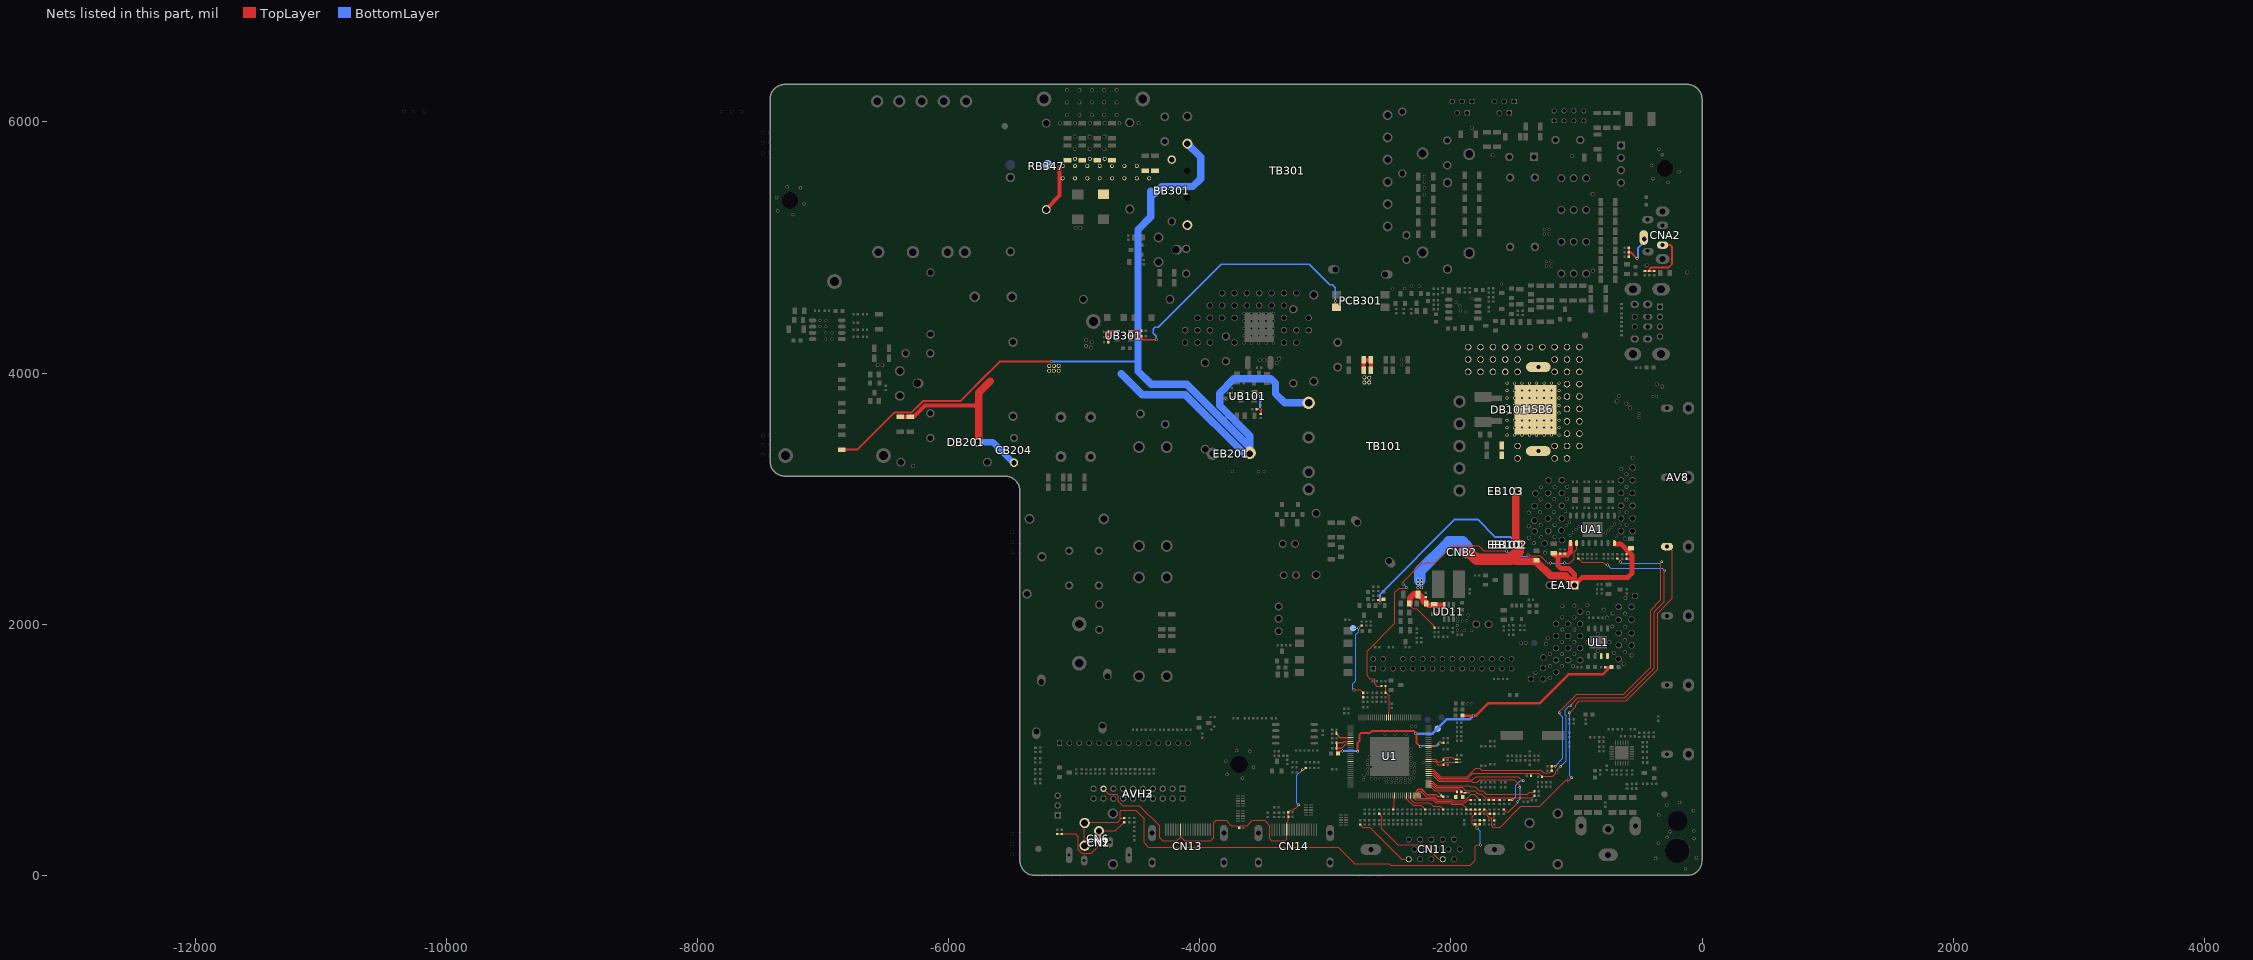
[diagram p0: the nets of this part, all layers, seen from the top]
# Altium PCB MISC84277.PcbDoc (part 7 of 15)
Units mil, origin at the board's own origin, x right, y up, seen from the top; angles counter-clockwise.
Board outline 7422.08 x 6299.21 mil, 2 copper layers (TopLayer, BottomLayer), stack 61.855 mil thick; 709 components, 395 nets, 2812 pads, 811 vias.

## Via types
v1: diameter 23.62, hole 15.75, TopLayer to BottomLayer, tented both sides, 437 vias
v2: diameter 19.68, hole 11.81, TopLayer to BottomLayer, tented both sides, 353 vias
v3: diameter 31.5, hole 23.62, TopLayer to BottomLayer, tented both sides, 16 vias
v4: diameter 31.5, hole 19.68, TopLayer to BottomLayer, tented both sides, 4 vias
v5: diameter 17.72, hole 9.84, TopLayer to BottomLayer, tented both sides, 1 vias

## Nets (pads, with @x,y where several pads share a name; then routed paths per layer and width w, separated by ;. In a path a pad name is that pad's centre, name@x,y a point inside that pad or via, vN(x,y) a via of type N, cw(c..) or ccw(c..) an arc to the next point about the centre after c; other vN are vias at no path point) (continued)
12V: C1.2 CA9.1 CA11.1 CA23.1 CA24.1 CD1.1 CD5.1 CD6.1 CD8.1 CD9.2 CD10.2 CNB2.2 DB101.2 EA1.1 EB101.1@-1464.92,2633.4 EB102.1@-1464.92,2633.4 EB103.1@-1465.89,3058.4 HSB6.1@-1304,3378.35 HSB6.2 pad.VIA5@-977.11,3419.43 pad.VIA5@-977.11,3517.85 pad.VIA5@-977.11,3616.28 pad.VIA5@-977.11,3714.7 pad.VIA5@-977.11,3813.13 pad.VIA5@-977.11,3911.55 pad.VIA5@-977.11,4009.98 pad.VIA5@-977.11,4108.4 pad.VIA5@-977.11,4206.83 pad.VIA5@-1075.53,3321 pad.VIA5@-1075.53,3419.43 pad.VIA5@-1075.53,3517.85 pad.VIA5@-1075.53,3616.28 pad.VIA5@-1075.53,3714.7 pad.VIA5@-1075.53,3813.13 pad.VIA5@-1075.53,3911.55 pad.VIA5@-1075.53,4009.98 pad.VIA5@-1075.53,4108.4 pad.VIA5@-1075.53,4206.83 pad.VIA5@-1139.59,3506 pad.VIA5@-1139.59,3565.05 pad.VIA5@-1139.59,3624.11 pad.VIA5@-1139.59,3683.16 pad.VIA5@-1139.59,3742.22 pad.VIA5@-1139.59,3801.27 pad.VIA5@-1139.59,3860.33 pad.VIA5@-1139.59,3919.38 pad.VIA5@-1173.96,3321 pad.VIA5@-1173.96,3419.43 pad.VIA5@-1173.96,4009.98 pad.VIA5@-1173.96,4108.4 pad.VIA5@-1173.96,4206.83 pad.VIA5@-1198.65,3506 pad.VIA5@-1198.65,3565.05 pad.VIA5@-1198.65,3624.11 pad.VIA5@-1198.65,3683.16 pad.VIA5@-1198.65,3742.22 pad.VIA5@-1198.65,3801.27 pad.VIA5@-1198.65,3860.33 pad.VIA5@-1198.65,3919.38 pad.VIA5@-1257.7,3506 pad.VIA5@-1257.7,3565.05 pad.VIA5@-1257.7,3624.11 pad.VIA5@-1257.7,3683.16 pad.VIA5@-1257.7,3742.22 pad.VIA5@-1257.7,3801.27 pad.VIA5@-1257.7,3860.33 pad.VIA5@-1257.7,3919.38 pad.VIA5@-1272.38,4206.83 pad.VIA5@-1316.76,3506 pad.VIA5@-1316.76,3565.05 pad.VIA5@-1316.76,3624.11 pad.VIA5@-1316.76,3683.16 pad.VIA5@-1316.76,3742.22 pad.VIA5@-1316.76,3801.27 pad.VIA5@-1316.76,3860.33 pad.VIA5@-1316.76,3919.38 pad.VIA5@-1370.81,4206.83 pad.VIA5@-1375.81,3506 pad.VIA5@-1375.81,3565.05 pad.VIA5@-1375.81,3624.11 pad.VIA5@-1375.81,3683.16 pad.VIA5@-1375.81,3742.22 pad.VIA5@-1375.81,3801.27 pad.VIA5@-1375.81,3860.33 pad.VIA5@-1375.81,3919.38 pad.VIA5@-1434.87,3506 pad.VIA5@-1434.87,3565.05 pad.VIA5@-1434.87,3624.11 pad.VIA5@-1434.87,3683.16 pad.VIA5@-1434.87,3742.22 pad.VIA5@-1434.87,3801.27 pad.VIA5@-1434.87,3860.33 pad.VIA5@-1434.87,3919.38 pad.VIA5@-1469.23,3321 pad.VIA5@-1469.23,3419.43 pad.VIA5@-1469.23,4009.98 pad.VIA5@-1469.23,4108.4 pad.VIA5@-1469.23,4206.83 pad.VIA5@-1493.92,3506 pad.VIA5@-1493.92,3565.05 pad.VIA5@-1493.92,3624.11 pad.VIA5@-1493.92,3683.16 pad.VIA5@-1493.92,3742.22 pad.VIA5@-1493.92,3801.27 pad.VIA5@-1493.92,3860.33 pad.VIA5@-1493.92,3919.38 pad.VIA5@-1552.98,3506 pad.VIA5@-1552.98,3565.05 pad.VIA5@-1552.98,3624.11 pad.VIA5@-1552.98,3683.16 pad.VIA5@-1552.98,3742.22 pad.VIA5@-1552.98,3801.27 pad.VIA5@-1552.98,3860.33 pad.VIA5@-1552.98,3919.38 pad.VIA5@-1567.66,4009.98 pad.VIA5@-1567.66,4108.4 pad.VIA5@-1567.66,4206.83 pad.VIA5@-1666.08,4009.98 pad.VIA5@-1666.08,4108.4 pad.VIA5@-1666.08,4206.83 pad.VIA5@-1764.51,4009.98 pad.VIA5@-1764.51,4108.4 pad.VIA5@-1764.51,4206.83 pad.VIA5@-1862.93,4009.98 pad.VIA5@-1862.93,4108.4 pad.VIA5@-1862.93,4206.83 pad.VIA5@-2234.25,2293.31 pad.VIA5@-2234.25,2323.31 pad.VIA5@-2234.25,2353.31 pad.VIA5@-2264.25,2293.31 pad.VIA5@-2264.25,2323.31 pad.VIA5@-2264.25,2353.31 R12V.1 RB123.2 RB124.2 RB131.1 RB135.1 RD1.1 UA1.1 UA1.8 UD11.3 | length 5785.1
  TopLayer w8: R12V.1@-2330.61,2164.35 -2330.61,2154.61 -2299,2123 -2271.05,2123 -2131.73,1983.68 RD1.1@-2131.73,1973
  TopLayer w15.75: v1(-2566.9,2167.23) -2566.93,2193.9 -2544.04,2193.9 RB131.1@-2537.4,2200.54 ; -1504.44,2672.93 -1485.57,2654.06 EB102.1@-1464.92,2633.4
  TopLayer w17: CA9.1@-602.27,2521.98 -575.52,2521.98
  TopLayer w40: CD8.1@-1181,2552 -1180,2551 CD8.1@-1168.03,2551 ; CD8.1@-1181,2563.97 CD8.1@-1168.03,2551 ; -1049,2609.97 -1049,2575 -1073,2551 CD8.1@-1168.03,2551 ; -1049.02,2609.98 UA1.1@-1049.02,2645.69 ; UA1.8@-688.5,2640.5 -648.5,2640.5 -559.5,2551.5 -559.5,2405 -590.5,2374 -953.24,2374 EA1.1@-1016.08,2311.16 -1016.08,2312.75 -1016.08,2397.78 -1063.18,2444.88 -1124.02,2444.88 -1146,2466.87 -1146,2528.97 CD8.1@-1168.03,2551
  TopLayer w45: CD1.1@-2215.7,2187.31 -2178.97,2150.58 -2105.54,2150.58 -2104.31,2149.35 -2065.2,2149.35
  TopLayer w50: R12V.1@-2326.77,2168.19 -2326.77,2206.69 -2295.23,2238.24 C1.2@-2261.81,2238.24 -2258.55,2238.24 -2215.7,2195.38 -2215.7,2187.31 -2215.7,2181.9 CD1.1@-2198.14,2164.33
  TopLayer w60: -1485.57,2558.01 -1485.57,2502 -1323,2502 -1206.83,2385.83 -1089.16,2385.83 EA1.1@-1016.08,2312.75 ; EB102.1@-1485.57,2654.06 -1485.57,3021
  TopLayer w90.55: CNB2.2@-1873.63,2567.74 -1847.27,2567.74 -1796.8,2517.28 -1526.31,2517.28 -1485.57,2558.01 -1464.92,2578.67 EB102.1@-1464.92,2633.4
  BottomLayer w15.75: v1(-2566.9,2167.23) -2566.9,2236.13 -1968.26,2834.77 -1787.37,2834.77 -1645.5,2692.9 -1524.42,2692.9 EB102.1@-1464.92,2633.4
  BottomLayer w90.55: -2250,2348.43 -2250,2421.72 -2016.21,2655.51 -1906.98,2655.51 -1873.63,2622.16 CNB2.2@-1873.63,2574.5
380V: CB204.2 DB201.K DB203.K EB201.1@-3602.55,3357 pad.VIA5@-2651.57,3925.2 pad.VIA5@-2651.57,3963.2 pad.VIA5@-2689.57,3925.2 pad.VIA5@-2689.57,3965.17 pad.VIA5@-4403.54,5551.18 pad.VIA5@-4501.97,5551.18 pad.VIA5@-4501.97,5649.61 pad.VIA5@-4600.39,5551.18 pad.VIA5@-4600.39,5649.61 pad.VIA5@-4698.82,5551.18 pad.VIA5@-4698.82,5649.61 pad.VIA5@-4757.87,5706.69 pad.VIA5@-4797.24,5551.18 pad.VIA5@-4797.24,5649.61 pad.VIA5@-4875.98,5706.69 pad.VIA5@-4895.67,5551.18 pad.VIA5@-4895.67,5649.61 pad.VIA5@-4994.09,5551.18 pad.VIA5@-4994.09,5649.61 pad.VIA5@-4994.09,5706.69 pad.VIA5@-5092.52,5551.18 pad.VIA5@-5092.52,5649.61 pad.VIA5@-5124,4018.9 pad.VIA5@-5124,4056.9 pad.VIA5@-5162,4018.9 pad.VIA5@-5162,4056.9 pad.VIA5@-5200,4018.9 pad.VIA5@-5200,4056.9 RB117.1 RB118.1 RB144.1 RB146.1 RB201.1 RB219.2 RB220.2 RB314.2 RB315.2 RB317.2 RB318.2 RB319.2 RB320.2 RB347.2 TB101.1 TB301.8@-4099.22,5828.04 TP-TDT.1 | length 11188.3
  TopLayer w15.75: RB201.1@-6853,3389.7 -6727.8,3389.7 -6432.46,3685.04 -6297.24,3685.04 -6204.72,3777.56 -5907.48,3777.56 ; -5679.13,4005.91 -5907.48,3777.56 ; v1(-5179.7,4090.6) -5594.44,4090.6 -5907.48,3777.56
  TopLayer w31.5: RB220.2@-6385.37,3651.1 -6280,3651.1 -6188.98,3742.13 -5795.28,3742.13 -5789.37,3736.22 ; -5772.86,3598.5 -5761.68,3587.32 ; RB347.2@-5221.58,5307.83 -5116.14,5413.28 -5116.14,5641.62 ; RB118.1@-2695.34,4022 -2695.34,4098.06 RB117.1@-2691.5,4101.91 ; RB117.1@-2695.34,4105.75 RB144.1@-2638.38,4105.75 RB146.1@-2638.38,4022
  TopLayer w59.06: DB201.K@-5761.68,3449 -5761.68,3587.32 -5761.68,3844.32 -5669.5,3936.5
  BottomLayer w15.75: v1(-5179.7,4090.6) -4493.37,4090.6
  BottomLayer w51.18: DB201.K@-5766.18,3449 -5647.82,3449 -5485.34,3286.52 CB204.2@-5480.13,3286.52
  BottomLayer w59.06: -4626.6,3996.2 -4459.14,3828.74 -4116.14,3828.74 EB201.1@-3644.41,3357 ; -4389.76,5283.01 -4389.76,5348.41 ; -4389.76,5446.85 -4389.76,5348.41 ; -4362.2,5429.13 -4305.12,5486.22 -4055.12,5486.22 -3992.13,5549.21 -3992.13,5720.94 TB301.8@-4099.22,5828.04 ; TB101.1@-3133.09,3762.99 -3323.99,3762.99 -3397.64,3836.64 -3397.64,3919.29 -3433.07,3954.72 -3728.35,3954.72 -3842.52,3840.55 -3842.52,3742.13 -3602.55,3502.16 -3602.55,3409.64 -4103.65,3910.74 -4387.8,3910.74 -4492.13,4015.07 -4492.13,5141.73 -4389.76,5244.09 -4389.76,5348.41
+1.8V_DDR: CF3.1 CF22.1 CF23.2 CF24.2 CL43.2 CL44.1 DDR_1V8.1 LF5.JP_2K U1.54 U1.106 UL1.7 UL1.8 | length 3202.1
  TopLayer w8: -2845,1039 -2834.96,1049.04 U1.106@-2800.46,1049.04 ; U1.54@-2178.42,1033.29 -2122.41,1033.29 -2099.7,1056 ; v1@-2086,1056 CF24.2@-2058.46,1056
  TopLayer w12: CF23.2@-2912.27,1012 -2872,1012 -2845,1039 ; CF3.1@-2901.19,970 -2881.19,990 v1(-2865,990)
  TopLayer w15: CF3.1@-2909.19,974 CF23.2@-2909.19,1003.92 ; v2@-2744.34,992.44 -2744.34,1053.69 -2727.34,1070.69 -2727.34,1122.98 -2715.32,1135 -2643.98,1135 -2627.98,1151 -2294.89,1151 v1@-2277.3,1133.4 ; v1@-2275,1129.6 -2275,1056 v1(-2244.5,1025.5)
  TopLayer w20: CF22.1@-1907.19,1273 v1(-1822,1273) -1800.36,1273 -1701.1,1372.26 -1292.45,1372.26 -1064.87,1599.84 -791.16,1599.84 -753,1638 -753,1659 CL44.1@-721.81,1659
  BottomLayer w15: v1(-2865,990) v2(-2741.9,990) ; v1@-2238.2,1031.8 -2110.2,1031.8 v1(-2086,1056)
  BottomLayer w20: v1@-2281.1,1129.1 -2146.9,1129.1 -2031,1245 -1850,1245 v1(-1822,1273)
  other v1: -2281.1,1129.6
AMP-OUTL: CF29.1 RA4.1 RF14.2 U1.41 | length 4030.7
  TopLayer w7: U1.41@-2178.42,828.57 -2140.57,828.57 -2084.53,772.53 -1865.67,772.53 -1825.7,812.5 -1777,812.5 ; -1781.86,812.5 -1777,812.5 ; CF29.1@-1363.27,791 CF29.1@-1363.27,793 -1363.27,812.23 -1363,812.5 ; v2@-1126.32,869.02 -1165.5,829.83 -1165.5,812.82 -1187.82,790.5 -1267.77,790.5 RF14.2@-1274.27,784 -1302.77,812.5 -1363,812.5 ; -1777,812.5 -1363,812.5
  TopLayer w8: v2(-1044,1352) -1044,1360.26 -988.42,1415.84 -615.08,1415.84 -380.74,1650.18 -380.74,2100.7 -302,2179.44 ; RA4.1@-986,2523.77 -955.14,2492.91 -789.64,2492.91 -768.73,2472 v1(-751.5,2472) ; -302,2180.85 v2@-302,2422
  BottomLayer w8: v2(-1125.34,869.02) -1080.84,913.51 -1080.84,1270.46 -1089.84,1279.46 -1089.84,1319.8 -1057.65,1352 v2(-1044,1352) ; v1(-751.5,2472) -727.02,2447.52 -316.52,2447.52 v2@-297,2428
  other v2: -296,2428
AMP-OUTR: CF30.1 RA12.1 RF15.2 U1.42 | length 3739.9
  TopLayer w7: U1.42@-2178.42,844.31 -2139.34,844.31 -2079.56,784.53 -1871.77,784.53 -1803.96,852.34 -1770.24,852.34 -1755.4,837.5 -1284.5,837.5 -1262.66,815.66 -1215.34,815.66 -1197.27,833.73 RF15.2@-1197.27,870 ; RF15.2@-1197.27,870 v2(-1169.85,870) RF15.2@-1197.27,870
  TopLayer w8: v2(-1139,1294) -1139,1302.03 -999.19,1441.84 -625.85,1441.84 -408.74,1658.95 -408.74,2112.3 -328,2193.04 -328,2490.65 v2(-322.16,2496.49) ; RA12.1@-675,2523.77 v1@-649.32,2498.09
  BottomLayer w8: v2(-1169.85,870) -1108.84,931.01 -1108.84,1258.44 -1139,1288.59 v2(-1139,1294) ; v1(-649.32,2494.33) -641.51,2486.52 -332.13,2486.52 v2(-322.16,2496.49)
AMP_STB: RA1.2 RA8.1 U1.81 | length 266
  TopLayer w6: RA8.1@-2520.27,1508 RA1.2@-2520.27,1454 -2517,1454 -2492.16,1429.16 -2492.16,1302.84 -2497.31,1297.69 U1.81@-2497.31,1257.7
AMP_STB/: RA8.2 UA1.2 | length 2788.6
  TopLayer w5: -2608,1563 -2608,1525.85 -2590.15,1508 RA8.2@-2553.73,1508
  TopLayer w6: -2608,1563 -2612,1567 -2647,1567 -2668.27,1588.27 -2668.27,1784.73 -2446,2007 -2446,2252.82 -2413.39,2285.43 -2360.24,2285.43 -2353.41,2292.26 v1(-2353.41,2291.8) ; v1(-2381.89,2320.87) -2381.89,2336.61 -2230.5,2488 -2128.72,2488 -1992.7,2624.02 -1777.56,2624.02 -1738.19,2584.65 v1(-1559.06,2584.65) ; v1(-1385.82,2553.14) -1376.68,2544 -1287,2544 -1229,2486 v1(-1208,2486) ; v1(-1094,2486) -1053,2486 -1018,2521 -1018,2577.88 -999.02,2596.87 UA1.2@-999.02,2645.69
  BottomLayer w6: v1(-2381.89,2320.87) -2353.41,2292.39 v1(-2353.41,2291.8) ; v1(-1559.06,2584.65) -1517.72,2543.31 -1393.7,2543.31 -1385.82,2551.18 v1(-1385.82,2553.14) ; v1(-1208,2486) v1(-1094,2486)
AUVAG: CF27.2 CF28.1 U1.33 | length 282.4
  TopLayer w8: U1.33@-2178.42,702.58 -2155.58,702.58 -2128.03,675.03 -1962.16,675.03 CF27.2@-1951.73,664.6 ; CF28.1@-1961.81,631 -1951.73,641.08 CF27.2@-1951.73,664.6 ; CF27.2@-1951.73,666.8 CF27.2@-1951.73,664.6
AUVRM: CF27.1 CF28.2 LF6.JP_1K U1.34 | length 362.7
  TopLayer w8: U1.34@-2178.42,718.33 -2152.95,718.33 -2122.65,688.03 -1933.93,688.03 -1918.9,673 CF27.1@-1918.27,673 ; CF28.2@-1906.19,631 -1906.9,631 -1918.27,642.37 CF27.1@-1918.27,673 ; LF6.JP_1K@-1888,658.4 -1903.67,658.4 CF27.1@-1918.27,673
AV1_LIN: CI3.1 U1.32 | length 440.9
  TopLayer w8: U1.32@-2245.34,635.65 -2245.34,622.38 -2238,615.03 -2138.42,615.03 -2114.38,591 -1997.06,591 -1985.9,579.84 -1884.77,579.84 -1863.88,600.73 CI3.1@-1844,600.73
AV1_LIN/: R3.2 RI4.2 RO15.1 | length 89.3
  TopLayer w8: RI4.2@-1692,490.27 RO15.1@-1655,490.27 R3.2@-1655,438
AV1_RIN: CI4.1 U1.31 | length 590.4
  TopLayer w8: U1.31@-2261.09,635.65 -2261.09,661.41 -2253.23,669.27 -2238.77,669.27 -2197.53,628.03 -2133.03,628.03 -2109,604 -1991.67,604 -1980.52,592.84 -1890.16,592.84 -1838,645 -1815,645 -1772,602 CI4.1@-1772,600.73
AV1_RIN/: R4.2 RI6.2 RO17.1 | length 88
  TopLayer w8: RI6.2@-1698,600.73 RO17.1@-1610,600.73
AV2_LIN: CI5.1 U1.36 | length 897.6
  TopLayer w7: U1.36@-2178.42,749.83 -2149.8,749.83 -2112.5,712.53 -1853.63,712.53 -1847.6,706.5 -1806.82,706.5 -1773.82,673.5 -1746.82,673.5 -1717.66,644.34 -1390.66,644.34 -1374,661 -1342.73,661 CI5.1@-1334.73,669
AV2_RIN: CI6.1 U1.35 | length 896.9
  TopLayer w7: U1.35@-2178.42,734.08 -2151.02,734.08 -2117.47,700.53 -1911.53,700.53 -1883.81,672.81 -1811.81,672.81 -1787.5,648.5 -1757.18,648.5 -1728.02,619.34 -1348.39,619.34 CI6.1@-1334.73,633
AV-OUTL: RO5.1 U1.39 | length 1066.4
  TopLayer w7: U1.39@-2178.42,797.07 -2144.07,797.07 -2095.53,748.53 -1834.59,748.53 -1828.56,742.5 -1789.5,742.5 -1771.5,760.5 -1749,760.5 -1548.5,760.5 -1494.5,760.5 -1452,718 v2(-1452,702)
  TopLayer w8: RO5.1@-1581,524.73 -1564.27,508 -1540.51,508 -1470,578.51 v2(-1470,588)
  BottomLayer w7: v2(-1470,588) -1449,609 v2@-1449,699
AV-OUTR: RO1.1 U1.40 | length 1031.2
  TopLayer w7: U1.40@-2178.42,812.82 -2142.85,812.82 -2090.56,760.53 -1824.87,760.53 -1798.4,787 -1792.42,787
  TopLayer w8: -1792.42,787 -1463,787 -1425,749 v2(-1425,752) ; RO1.1@-1537,600.73 v2@-1511.27,600.73
  BottomLayer w8: v2(-1511,601) -1484,628 -1484,717 -1449,752 v2(-1425,752)
AV_IN: CI1.1 U1.27 | length 324.9
  TopLayer w7: U1.27@-2324.08,635.65 -2324.08,610.95 -2303.07,589.93 -2303.07,589.88 -2292.72,579.53 -2171.53,579.53 -2142.71,550.71 -2086.98,550.71 CI1.1@-2060,523.73
AVDD5V_MHL: U1.115 | length 0.7
  TopLayer w6: U1.115@-2800.97,907.81 U1.115@-2800.46,907.31
AVDD_AU33: CF13.2 LF2.JP_1K U1.30 | length 279.5
  TopLayer w8: U1.30@-2276.84,635.65 -2276.84,668.29
  TopLayer w12: -2276.84,668.29 -2259.85,685.27 -2232.15,685.27 -2189.9,643.03 -2120.03,643.03 -2102,625 CF13.2@-2062,625
AVDD_DADC: CF14.2 LF3.JP_1K U1.46 | length 247.5
  TopLayer w8: U1.46@-2178.42,907.31 -2126.97,907.31 -2099.67,880 -2059.47,880 CF14.2@-2058.46,881 -2058.46,888.54 -2046,901 LF3.JP_1K@-1955.3,901
AVDD_DDR_DATA: CF25.2 LF5.JP_1K U1.105 | length 127.1
  TopLayer w8: -2840,1064.79 U1.105@-2800.46,1064.79
  TopLayer w12: CF25.2@-2912.27,1047.73 CF25.2@-2912.27,1055 ; CF25.2@-2912.27,1059 CF25.2@-2912.27,1055 ; -2840,1064.79 -2851.21,1064.79 -2861,1055 CF25.2@-2912.27,1055
AVDD_DMPLL: CF12.2 LF1.JP_1K U1.47 | length 255.9
  TopLayer w8: U1.47@-2178.42,923.05 -2124.34,923.05 -2104.28,903 -2076.47,903 CF12.2@-2058.46,921 -2058.46,927.54 -2045,941 -1988,941 -1973.4,926.4 LF1.JP_1K@-1956.4,926.4
BL_ON: BL_ON.1 CG1.1 RB386.2 RG1.1 | length 708.6
  TopLayer w6: v1(-2771.65,1476.38) -2721.11,1476.38 CG1.1@-2698.73,1454 RG1.1@-2698.73,1417 ; v1(-2736.09,1968.56) -2715.4,1989.25 RB386.2@-2711.79,1989.25
  BottomLayer w6: BL_ON.1@-2777.56,1968.5 -2736.15,1968.5 v1(-2736.09,1968.56) -2736.09,1941.07 -2757,1920.17 -2757,1550.09 -2781.5,1525.59 -2781.5,1486.22 v1(-2771.65,1476.38)
BRO: RB104.2 RB143.2 UB101.3 | length 244.7
  TopLayer w15.75: UB101.3@-3565.35,3851.9 -3542.85,3851.9 v1(-3519.68,3828.73) ; RB104.2@-3548.27,3713.5 v1@-3520.59,3713.5 ; v1@-3516.4,3713.5 v1@-3520.59,3713.5 ; RB143.2@-3513,3675.23 -3513,3705.91 v1(-3519.68,3712.59) v1@-3520.59,3713.5
  BottomLayer w15.75: v1(-3519.68,3712.59) v1(-3519.68,3828.73)
BRO1: RB304.1 UB301.3 | length 89.7
  TopLayer w15.75: UB301.3@-4551.9,4334.65 -4467.8,4334.65 RB304.1@-4463.81,4338.63
CEC: AVH2.17 AVH3.17 CH7.2 CH10.2 CN13.13 CN14.13 DH10.K RH13.2 | length 2784.1
  TopLayer w6: AVH2.17@-4767.74,689.7 -4723.44,645.4 -4662.7,645.4 -4648.4,631.1 -4648.4,589.9 -4614.6,556.1 -4483.37,556.1 -4321.1,393.83 -4321.1,300.13 -4294.77,273.8 -4183,273.8 -4153.55,303.25 ; CN13.13@-4153.55,364.62 -4153.55,306.26 -4121.78,274.5 -3912.53,274.5 -3888,299.03 -3888,420.05 -3871,437.05 -3788.4,437.05 -3748.01,396.67 -3705,396.67 -3689.87,381.53 -3688.65,380.32 CH10.2@-3686.43,378.1 ; CH10.2@-3691.4,380 -3688.97,380 -3672.3,396.67 -3621.55,396.67 -3581.17,437.05 -3484.05,437.05 -3442.5,395.5 -3442.5,291.5 -3427.69,276.69 -3318.31,276.69 -3307.09,287.91 CN14.13@-3307.09,364.62 -3307.09,420.93 -3294.63,433.39 -3294.74,433.5 CH7.2@-3294.74,466.29 ; CH7.2@-3294.96,467.23 DH10.K@-3294.96,503.7 ; DH10.K@-3294.96,505.54 DH10.K@-3294.96,503.7 ; v2@-3216.24,562.9 v2(-3214,562.9) -3214,560.11 -3238.1,536.01 -3243.12,536.01 -3256.61,522.52 -3276.14,522.52 DH10.K@-3294.96,503.7 ; v2@-3182,841.7 -3169.83,841.7 RH13.2@-3156.43,855.1
  BottomLayer w6: v2(-3214,562.9) -3213.96,562.94 -3227,575.98 -3227,796.7 v2@-3182,841.7
  other v2: -3183.2,841.7
COAX_OUT: CN1.1 CN2.1 CO6.1 CO7.1 RO6.1 | length 831
  TopLayer w8: CO6.1@-5136.7,330.07 -4991.07,330.07 -4969.3,308.3 -4969.3,203 -4942,175.7 -4863.2,175.7 -4803.22,235.68 CN2.1@-4803.22,354.18 -4671.99,354.18 RO6.1@-4603.2,422.97
COMP: CB301.2 PCB301.4 UB301.2 | length 2210.7
  TopLayer w11.81: CB301.2@-4463.81,4295.33 -4463.81,4273.03 -4456.53,4265.75 v1(-4346.46,4265.75) ; PCB301.4@-2921,4535.37 v1(-2921,4574)
  TopLayer w15.75: UB301.2@-4551.9,4297.24 CB301.2@-4465.73,4297.24
  BottomLayer w11.81: v1(-4346.46,4265.75) -4346.46,4293.31 -4372.22,4319.07 -4372.22,4349.29 -4357.16,4364.35 -4330.99,4364.35 -3829.07,4866.27 -3127.62,4866.27 -2964.07,4702.72 -2942.85,4702.72 -2921,4680.87 v1(-2921,4574)
CS: CB303.1 RB303.1 RB305.1 UB301.4 | length 158.7
  TopLayer w15.75: RB303.1@-4728.68,4244.24 CB303.1@-4728.68,4287.55 RB305.1@-4728.68,4330.86 -4724.89,4334.65 UB301.4@-4658.19,4334.65
CVBS_IN_OUT: AV8.1 RI2.1 RO2.1 | length 3496
  TopLayer w8: RO2.1@-1771,490.27 -1767.46,490.27 -1730.87,526.87 -1713,509 -1713,476 -1696,459 -1681,459 -1677,455 -1677,395 -1667,385 -1608.35,385 -1442.35,551 -1293.81,551 -1086.05,758.76 -1056.51,758.76 v2(-1036.82,778.45) ; v2(-1058,1294) -1055.62,1294 -1007.01,1342.61 -1007.01,1360.49 -977.65,1389.84 -604.31,1389.84 -352.74,1641.41 -352.74,2089.1 -236.32,2205.53 -236.32,2584.5 -269.93,2618.11 AV8.1@-279.53,2618.11
  BottomLayer w8: v2(-1058,1294) -1052.84,1288.84 -1052.84,1232 ; -1052.84,1266.88 -1052.84,1232 ; v2@-1036.82,781.58 v2(-1036.82,778.45) -1052.84,794.47 -1052.84,1232
CVBS_OUT: CO9.2 RO2.2 RO12.1 RO13.2 U1.29 | length 590.8
  TopLayer w7: U1.29@-2292.59,635.65 -2292.59,611.98 -2283.14,602.53 -2143.59,602.53 -2119.56,578.5 -2003.2,578.5 -1992.05,567.34 -1908.34,567.34 -1880,539 CO9.2@-1880,523.73 RO13.2@-1808,523.73 RO2.2@-1771,523.73
CVBS_OUT/: CN6.4 CN6.5 DU1.K RO6.2 RO13.1 RO16.2 | length 4176.3
  TopLayer w8: CN6.4@-4921.26,236.07 -4921.26,417.17 -4914.13,424.3 -4653.9,424.3 -4632.3,445.9 -4632.3,509.5 -4624.3,517.5 -4511.38,517.5 -4444.5,450.62 -4444.5,258.32 -4410.68,224.5 -2897.96,224.5 -2766.52,93.06 -2489.74,93.06 -2479.06,82.38 -1844.62,82.38 -1805.35,121.65 -1805.35,226.65 -1790,242 v1(-1766.5,242) ; -4630.17,456.43 RO6.2@-4603.2,456.43 ; RO13.1@-1808,490.27 -1832,466.27 -1832,412 -1824.54,404.54 DU1.K@-1797.5,404.54 ; v1@-1797.5,382.49 DU1.K@-1797.5,404.54 ; RO16.2@-1778,404.54 DU1.K@-1797.5,404.54
  BottomLayer w8: v1(-1792.88,377.87) -1766.5,351.49 v1(-1766.5,242)
D: BB301.2 TB301.11@-4099.22,5178.43
DDC_SCL: CN11.15 RF11.2 | length 502.3
  TopLayer w6: RF11.2@-2722,405.27 -2722,403 -2703,384 -2648,384 -2392,128 CN11.15@-2335.83,128
DDC_SDA: CN11.12 RF10.2 | length 740.7
  TopLayer w6: RF10.2@-2572,491.27 -2552,471.27 -2552,370 -2424,242 -2170,242 -2154,226 -2154,184.5 -2097.5,128 CN11.12@-2065.36,128
DVD_DET: U1.82
DVD_IR/: U1.80
DVD_ON: U1.53
DVDD_DDR: CF21.2 LF4.JP_1K U1.103 | length 125.1
  TopLayer w8: -2831,1096.28 U1.103@-2800.46,1096.28
  TopLayer w12: CF21.2@-2912.27,1127 -2881.55,1096.28 -2831,1096.28 ; CF21.2@-2911.77,1125.5 CF21.2@-2911.5,1125.5 ; CF21.2@-2911.77,1128 CF21.2@-2911.52,1127.75
EP_L: CA61.1 CNA2.3 RA14.2 RA28.1 | length 390.8
  TopLayer w15: RA28.1@-583.49,4924.87 CA61.1@-583.49,4961.5 RA14.2@-583.49,4997.8 ; CA61.1@-583.49,4961.69 -566.99,4961.69 v1(-520,4914.7) ; CNA2.3@-460.63,5033.74 -460.63,5067.08 CNA2.3@-443.21,5084.5
  BottomLayer w15: v1(-520,4914.7) -510.88,4923.82 -510.88,4994.58 -460.63,5044.82 CNA2.3@-460.63,5067.08
EP_R: CA60.1 CNA2.2 RA9.2 RA23.1 | length 517.8
  TopLayer w15: RA9.2@-451.16,4814.25 CA60.1@-418.76,4814.25 ; CA60.1@-419.79,4813.22 CA60.1@-418.76,4814.25 ; RA23.1@-382.79,4814.25 CA60.1@-418.76,4814.25 ; CNA2.2@-314.96,5002.91 -314.96,5019.84 -252.21,5019.84 -238.87,5006.5 -238.87,4868.83 -267.7,4840 -408.8,4840 -418.1,4830.7 -418.1,4814.91 CA60.1@-418.76,4814.25
EX_AV: RI1.1 RO16.1 | length 37
  TopLayer w8: RO16.1@-1771,439.73 RI1.1@-1734,439.73
GIN0N: CF31.1 U1.19 | length 115
  TopLayer w8: CF31.1@-2460,524.73 -2460,542 -2450.07,551.93 U1.19@-2450.07,635.65
GIN1N: CF34.1 U1.25 | length 211.6
  TopLayer w6: U1.25@-2355.58,635.65 -2355.58,610.57 -2302.04,557.03 -2238.3,557.03 CF34.1@-2205,523.73